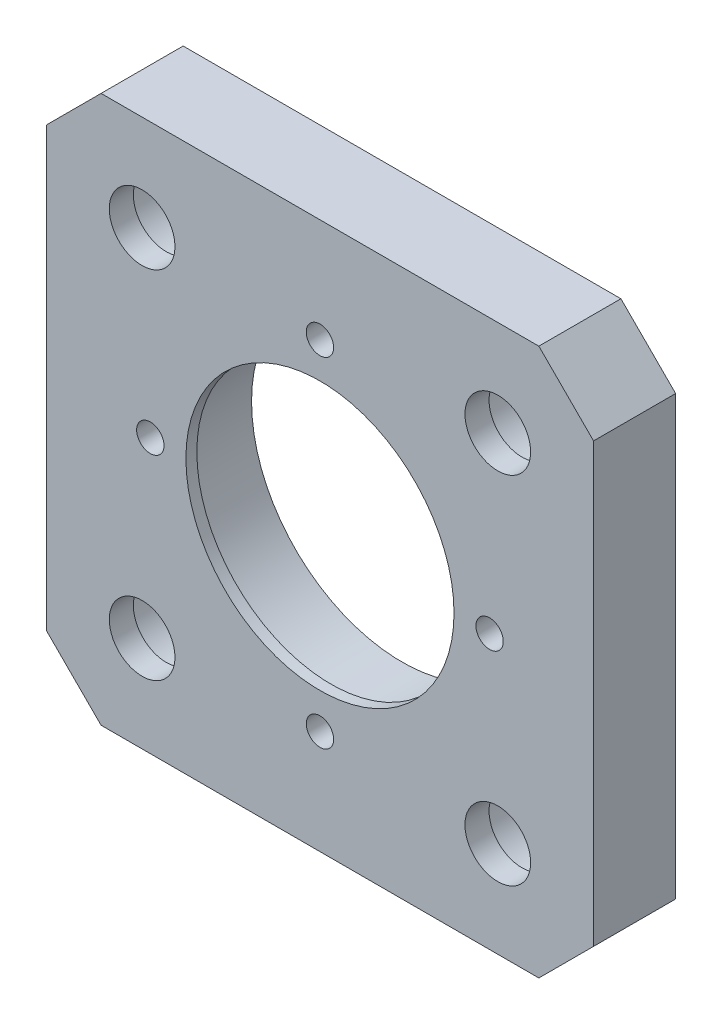
from build123d import *

# Parameters (mm, degrees)
SKETCH_1_W                    = 100
SKETCH_1_H                    = 100
EXTRUDE_1_DEPTH               = 15
HOLE_WIZARD_M10_1_D           = 12
HOLE_WIZARD_M10_1_CBORE_D     = 18
HOLE_WIZARD_M10_1_CBORE_DEPTH = 10.6
CHAMFER_1_SIZE                = 10
SKETCH_11_R                   = 27.5
CUT_EXTRUDE_4_DEPTH           = 13
HOLE_WIZARD_M6_1_D            = 5
HOLE_WIZARD_M6_1_DEPTH        = 15
HOLE_WIZARD_M6_1_TIP          = 1.502151548
SKETCH_14_R                   = 24.5
CUT_EXTRUDE_5_DEPTH           = 72.895757872


with BuildPart() as part:
    # 草图1 → 凸台-拉伸1 (new body)
    with BuildSketch(Plane.XY):
        Rectangle(SKETCH_1_W, SKETCH_1_H)
    extrude(amount=EXTRUDE_1_DEPTH)

    # M10 六角凹头螺钉的柱形沉头孔1 (through all)
    with Locations(Plane(origin=(0, 0, 0), x_dir=(-1, 0, 0), z_dir=(0, 0, -1))):
        with Locations((-32.5, 32.5), (32.5, 32.5), (32.5, -32.5), (-32.5, -32.5)):
            CounterBoreHole(HOLE_WIZARD_M10_1_D / 2, HOLE_WIZARD_M10_1_CBORE_D / 2, HOLE_WIZARD_M10_1_CBORE_DEPTH)

    # 倒角1
    chamfer_1_edges = [part.edges().sort_by_distance(p)[0] for p in [
        (50, -50, 7.5),
        (-50, -50, 7.5),
        (-50, 50, 7.5),
        (50, 50, 7.5),
    ]]
    chamfer(chamfer_1_edges, length=CHAMFER_1_SIZE)

    # 草图11 → 切除-拉伸4 (cut)
    with BuildSketch(Plane(origin=(0, 0, 0), x_dir=(-1, 0, 0), z_dir=(0, 0, -1))):
        Circle(SKETCH_11_R)
    extrude(amount=-CUT_EXTRUDE_4_DEPTH, mode=Mode.SUBTRACT)

    # M6 螺纹孔1
    with Locations(Plane(origin=(0, 0, 0), x_dir=(-1, 0, 0), z_dir=(0, 0, -1))):
        with Locations((0, 31), (31, 0), (0, -31), (-31, 0)):
            Hole(HOLE_WIZARD_M6_1_D / 2, depth=HOLE_WIZARD_M6_1_DEPTH)
            with Locations((0, 0, -(HOLE_WIZARD_M6_1_DEPTH + HOLE_WIZARD_M6_1_TIP / 2))):  # 118° drill point
                Cone(0, HOLE_WIZARD_M6_1_D / 2, HOLE_WIZARD_M6_1_TIP, mode=Mode.SUBTRACT)

    # 草图14 → 切除-拉伸5 (cut, through all)
    with BuildSketch(Plane(origin=(0, 0, 13), x_dir=(-1, 0, 0), z_dir=(0, 0, -1))):
        Circle(SKETCH_14_R)
    extrude(amount=-CUT_EXTRUDE_5_DEPTH, mode=Mode.SUBTRACT)


solid = part.part
